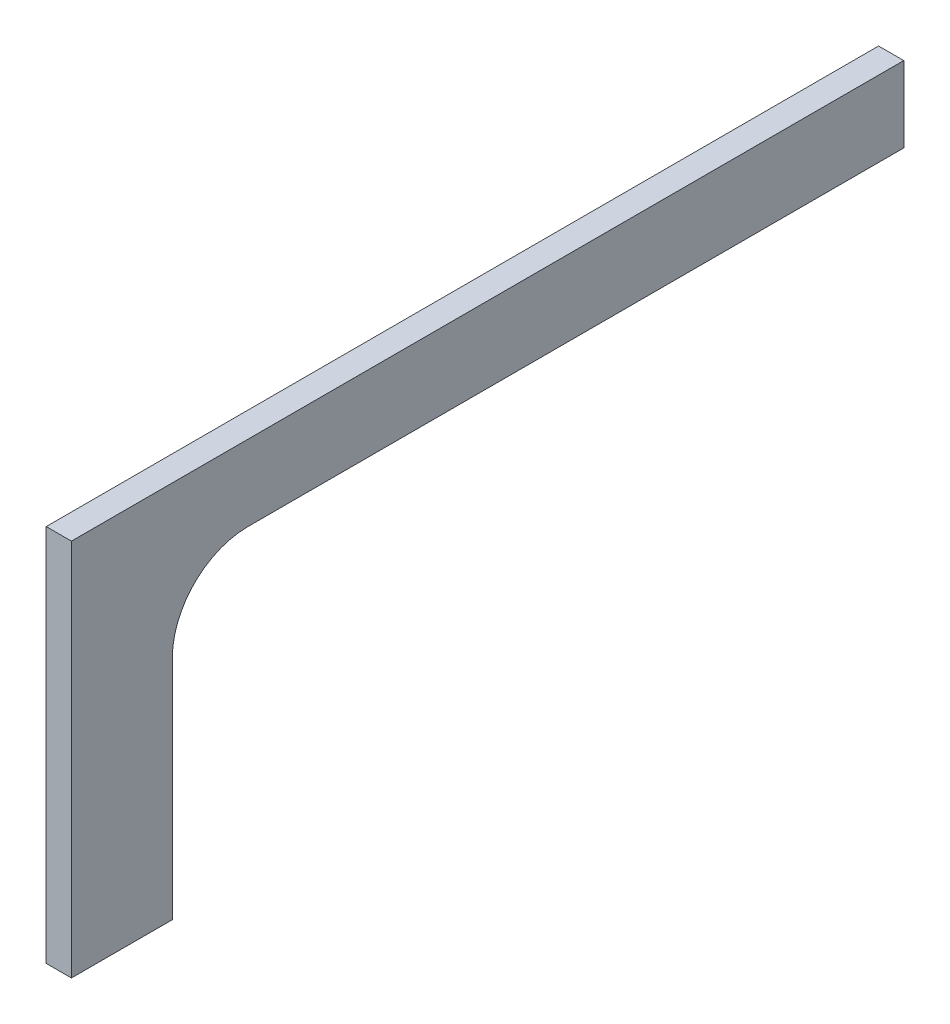
SolidWorks part; units mm, degrees
ref_plane "前视基准面" through (0, 0, 0) normal (0, 0, 1) x (1, 0, 0)
ref_plane "上视基准面" through (0, 0, 0) normal (0, 1, 0) x (1, 0, 0)
ref_plane "右视基准面" through (0, 0, 0) normal (1, 0, 0) x (0, 0, -1)
sketch "草图1" plane through (0, 0, 0) normal (0, 0, 1) x (1, 0, 0)
  line L1 (-10, -150) -> (10, -150)
  line L2 (-10, -150) -> (-10, 150)
  line L3 (-10, 150) -> (10, 150)
  line L4 (10, -150) -> (10, 150)
  line L5 (-10, -150) -> (10, 150) construction
  line L6 (-10, 150) -> (10, -150) construction
  point P0 (0, 0)
  dimension "D1" = 20
  dimension "D2" = 300
extrude "凸台-拉伸1" add sketch "草图1" along normal mid plane 660
sketch "草图2" plane through (10, 0, 0) normal (1, 0, 0) x (0, 0, -1)
  line L0 (330, -150) -> (330, 150) construction
  line L1 (330, 90) -> (-250, 90)
  line L2 (330, 90) -> (330, -150)
  line L3 (330, -150) -> (-250, -150)
  line L4 (-250, 90) -> (-250, -150)
  line L5 (-330, -150) -> (330, -150) construction
  dimension "D1" = 580
  dimension "D2" = 240
extrude "切除-拉伸1" cut sketch "草图2" against normal through all
fillet "圆角1" radius 60 1 edges at (0, 90, 250)
